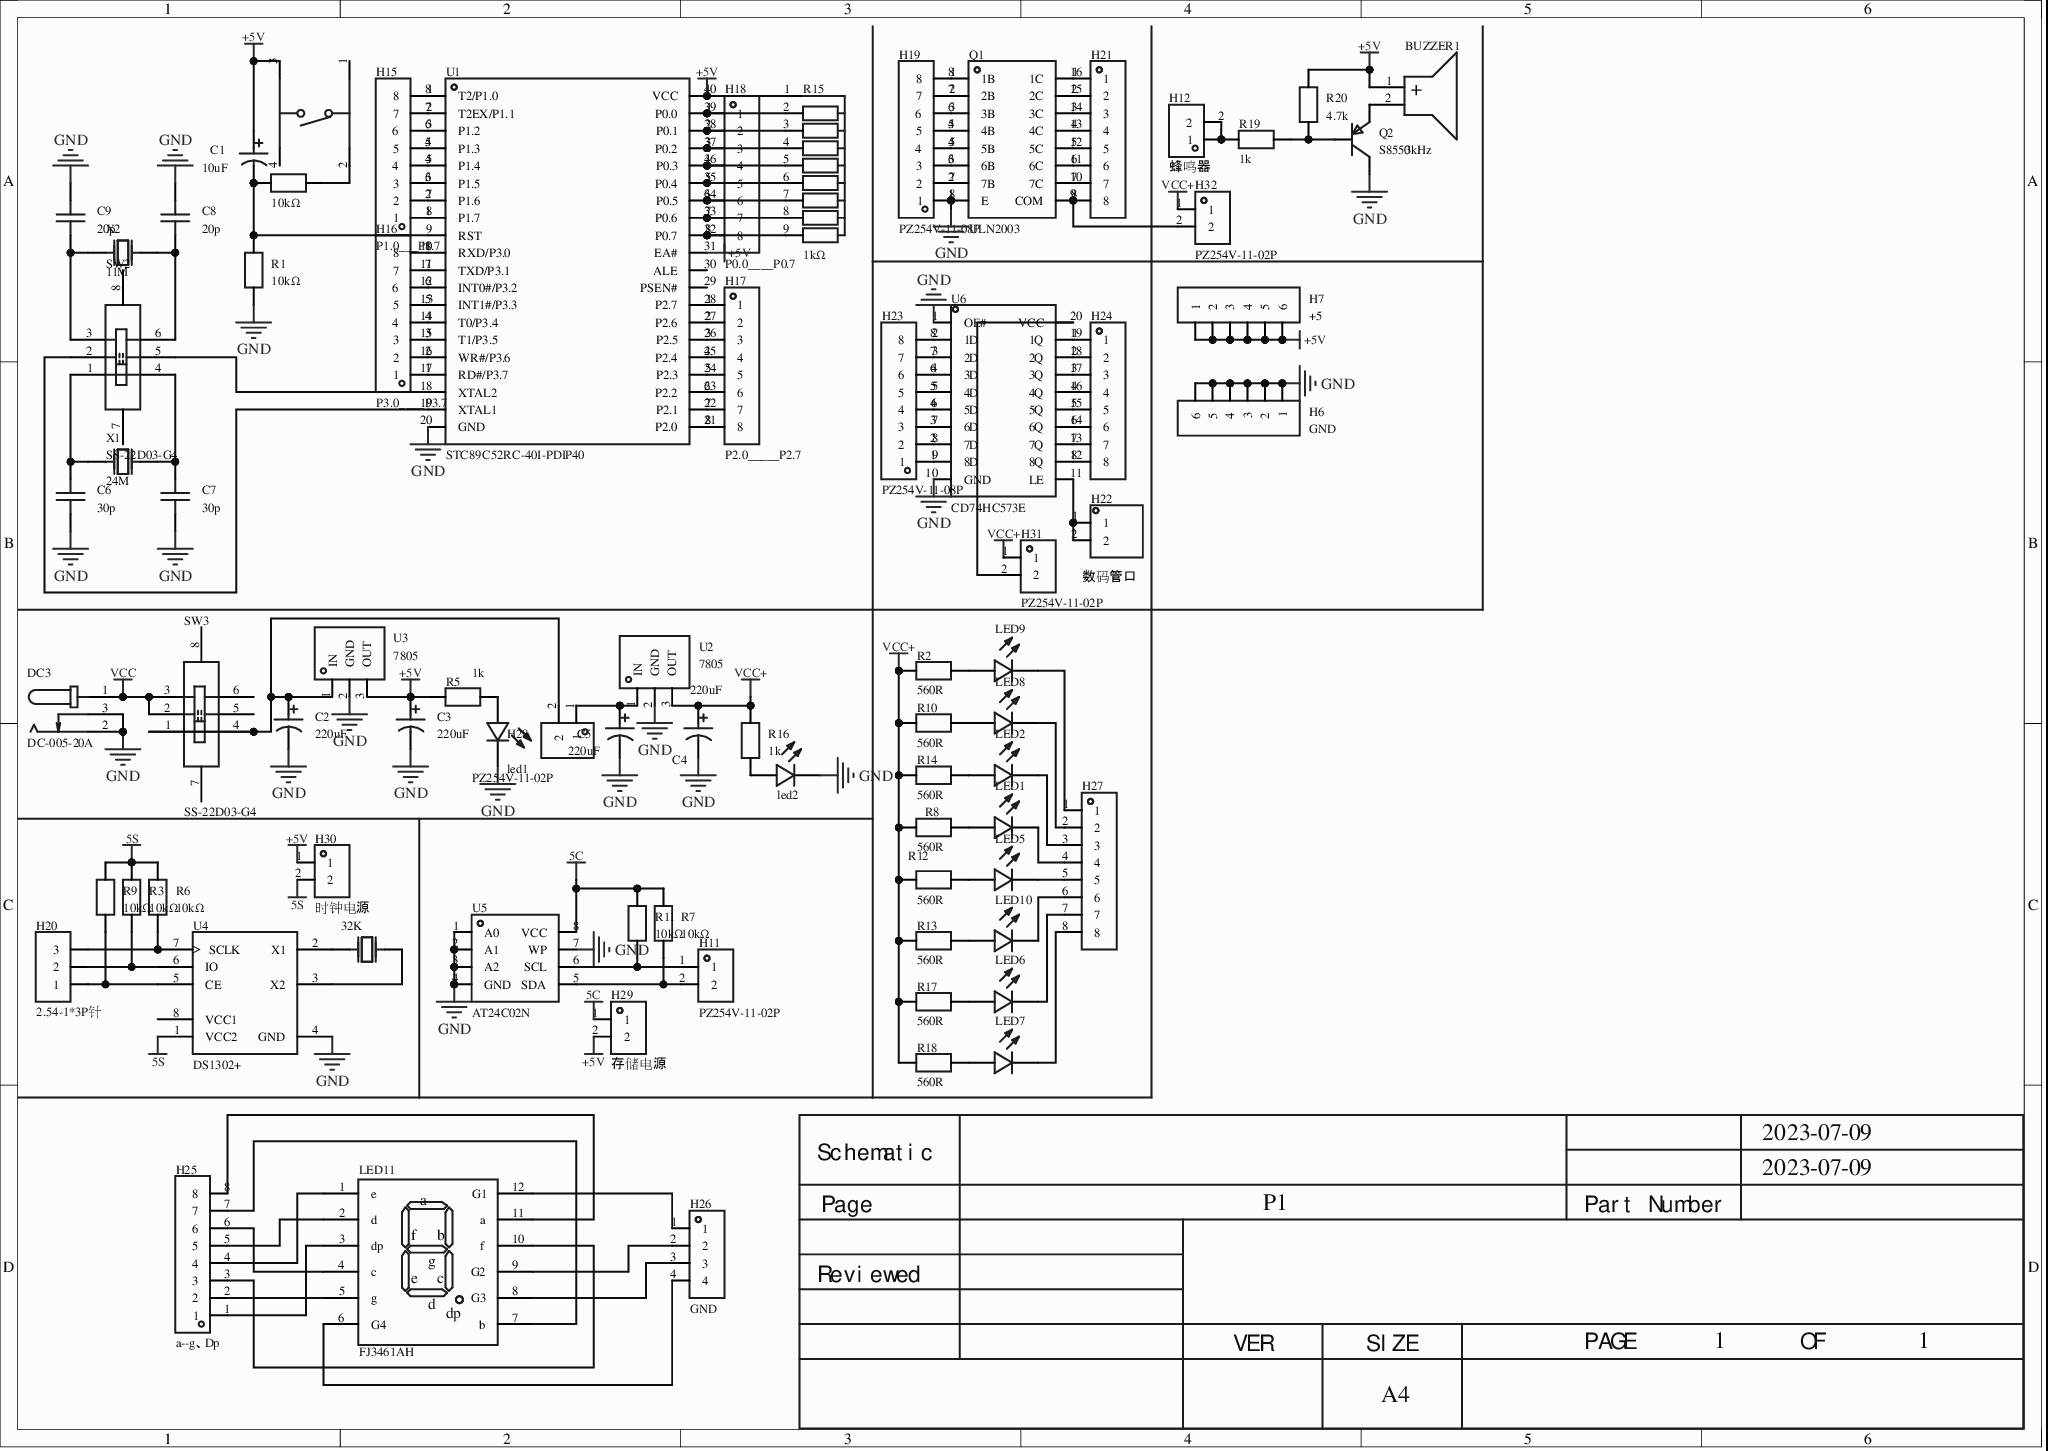
[diagram p0: MISC49922-3.schdoc]
# Altium project MISC49922-2.PrjPcb
1 sheet, 78 parts. Net scope: global (net labels, ports and power ports of the same name join across sheets).
Board file: MISC49922.pcbdoc

## Sheet MISC49922-3.schdoc
size 297 x 210 mm; Version: V1.0; @Project Name: MISC49922; @Page Count: 1; @Update Date: 2023-07-09; @Create Date: 2023-07-09; @Schematic Name: MISC49922; @Page No: 1

### Parts
BUZZER1  3kHz  [BUZ-TH_BD9.0-P5.00-D0.6-FD]
C1  10uF  [CAP-TH_BD5.0-P2.00-D0.8-FD]
C2  220uF  [CAP-TH_BD8.0-P3.50-D0.6-FD]
C3  220uF  [CAP-TH_BD8.0-P3.50-D0.6-FD]
C4  220uF  [CAP-TH_BD8.0-P3.50-D0.6-FD]
C5  220uF  [CAP-TH_BD8.0-P3.50-D0.6-FD]
C6  30p  [CAP-TH_L5.0-W5.0-P2.54-D1.0]
C7  30p  [CAP-TH_L5.0-W5.0-P2.54-D1.0]
C8  20p  [CAP-TH_L5.0-W5.0-P2.54-D1.0]
C9  20p  [CAP-TH_L5.0-W5.0-P2.54-D1.0]
DC3  DC-005-20A  [DC-IN-TH_DC-005-20A]
H6  GND  [HDR-TH_6P-P2.54-V-M-1]
H7  +5  [HDR-TH_6P-P2.54-V-M-1]
H11  PZ254V-11-02P  [HDR-TH_2P-P2.54-V-M]
H12  蜂鸣器  [HDR-TH_2P-P2.54-V-M]
H15  P1.0___P1.7  [HDR-TH_8P-P2.54-V-M]
H16  P3.0____P3.7  [HDR-TH_8P-P2.54-V-M]
H17  P2.0_____P2.7  [HDR-TH_8P-P2.54-V-M]
H18  P0.0____P0.7  [HDR-TH_8P-P2.54-V-M]
H19  PZ254V-11-08P  [HDR-TH_8P-P2.54-V-M]
H20  2.54-1*3P针  [HDR-TH_3P-P2.54-V-M-1]
H21  PZ254V-11-08P  [HDR-TH_8P-P2.54-V-M]  (value not drawn)
H22  数码管口  [HDR-TH_2P-P2.54-V-M-1]
H23  PZ254V-11-08P  [HDR-TH_8P-P2.54-V-M]
H24  PZ254V-11-08P  [HDR-TH_8P-P2.54-V-M]  (value not drawn)
H25  a--g、Dp  [HDR-TH_8P-P2.54-V-M]
H26  GND  [HDR-TH_4P-P2.54-V-M]
H27  PZ254V-11-08P  [HDR-TH_8P-P2.54-V-M]  (value not drawn)
H28  PZ254V-11-02P  [HDR-TH_2P-P2.54-V-M]
H29  存储电源  [HDR-TH_2P-P2.54-V-M]
H30  时钟电源  [HDR-TH_2P-P2.54-V-M]
H31  PZ254V-11-02P  [HDR-TH_2P-P2.54-V-M]
H32  PZ254V-11-02P  [HDR-TH_2P-P2.54-V-M]
LED1  204-10SURD/S530-A3-L  [LED-TH_BD3.0-P2.54-FD]  (value not drawn)
LED2  204-10SURD/S530-A3-L  [LED-TH_BD3.0-P2.54-FD]  (value not drawn)
LED3  led1  [LED-TH_BD3.0-P2.54-FD]
LED4  led2  [LED-TH_BD3.0-P2.54-FD]
LED5  204-10SURD/S530-A3-L  [LED-TH_BD3.0-P2.54-FD]  (value not drawn)
LED6  204-10SURD/S530-A3-L  [LED-TH_BD3.0-P2.54-FD]  (value not drawn)
LED7  204-10SURD/S530-A3-L  [LED-TH_BD3.0-P2.54-FD]  (value not drawn)
LED8  204-10SURD/S530-A3-L  [LED-TH_BD3.0-P2.54-FD]  (value not drawn)
LED9  204-10SURD/S530-A3-L  [LED-TH_BD3.0-P2.54-FD]  (value not drawn)
LED10  204-10SURD/S530-A3-L  [LED-TH_BD3.0-P2.54-FD]  (value not drawn)
LED11  FJ3461AH  [LED-SEG-TH_12P-L30.0-W14.0-P2.54-S10.16-BL]
Q1  ULN2003  [DIP-16_L19.8-W6.5-P2.54-LS7.6-BL]
Q2  S8550  [TO-92-3_L4.9-W3.7-P1.27-L]
R1  10kΩ  [RES-TH_BD2.4-L6.3-P10.30-D0.6]
R2  560R  [RES-TH_BD2.4-L6.3-P10.30-D0.6]
R3  10kΩ  [RES-TH_BD2.4-L6.3-P10.30-D0.6]
R4  10kΩ  [RES-TH_BD2.4-L6.3-P10.30-D0.6]
R5  1k  [RES-TH_BD2.4-L6.3-P10.30-D0.6]
R6  10kΩ  [RES-TH_BD2.4-L6.3-P10.30-D0.6]
R7  10kΩ  [RES-TH_BD2.4-L6.3-P10.30-D0.6]
R8  560R  [RES-TH_BD2.4-L6.3-P10.30-D0.6]
R9  10kΩ  [RES-TH_BD2.4-L6.3-P10.30-D0.6]
R10  560R  [RES-TH_BD2.4-L6.3-P10.30-D0.6]
R11  10kΩ  [RES-TH_BD2.4-L6.3-P10.30-D0.6]
R12  560R  [RES-TH_BD2.4-L6.3-P10.30-D0.6]
R13  560R  [RES-TH_BD2.4-L6.3-P10.30-D0.6]
R14  560R  [RES-TH_BD2.4-L6.3-P10.30-D0.6]
R15  1kΩ  [RES-ARRAY-TH_9P-L22.8-W3.00-P2.54]
R16  1k  [RES-TH_BD2.4-L6.3-P10.30-D0.6]
R17  560R  [RES-TH_BD2.4-L6.3-P10.30-D0.6]
R18  560R  [RES-TH_BD2.4-L6.3-P10.30-D0.6]
R19  1k  [RES-TH_BD2.4-L6.3-P10.30-D0.6]
R20  4.7k  [RES-TH_BD2.4-L6.3-P10.30-D0.6]
SW1  TS-1095-A7B2-D1  [SW-TH_4P-L6.0-W6.0-P4.50-LS6.5]  (value not drawn)
SW2  SS-22D03-G4  [SW-TH_SS-22D03-G4]
SW3  SS-22D03-G4  [SW-TH_SS-22D03-G4]
U1  STC89C52RC-40I-PDIP40  [DIP-40_L52.0-W13.7-P2.54-LS15.2-BL]
U2  7805  [TO-220-3_L10.0-W4.5-P2.54-L]
U3  7805  [TO-220-3_L10.0-W4.5-P2.54-L]
U4  DS1302+  [DIP-8_L9.8-W6.6-P2.54-LS7.6-BL]
U5  AT24C02N  [DIP-8_L9.2-W6.3-P2.54-LS7.62-BL]
U6  CD74HC573E  [DIP-20_L26.8-W6.4-P2.54-LS7.6-BL]
X1  24M  [HC-49US_L11.5-W4.5-P4.88]
X2  11M  [HC-49US_L11.5-W4.5-P4.88]
X3  32K  [HC-49US_L11.5-W4.5-P4.88]

### Nets
5C: H29.1 R7.2 R11.2 U5.8(VCC)
5S: H30.2 R3.2 R6.2 R9.2 U4.1(VCC2)
+5V: BUZZER1.1(+) C1.1 C3.1 H7.1 H7.2 H7.3 H7.4 H7.5 H7.6 H29.2 H30.1 R5.1 R15.1 R20.2 SW1.3 U1.31(EA#) U1.40(VCC) U3.3(OUT)
GND: C2.2 C3.2 C4.2 C5.2 C6.1 C7.1 C8.2 C9.1 DC3.2 DC3.3 H6.1 H6.2 H6.3 H6.4 H6.5 H6.6 H19.1 LED3.2(K) LED4.2(K) Q1.8(E) Q2.3(C) R1.1 U1.20(GND) U2.2(GND) U3.2(GND) U4.4(GND) U5.1(A0) U5.2(A1) U5.3(A2) U5.4(GND) U5.7(WP) U6.1(OE#) U6.10(GND)
VCC: DC3.1 SW3.2 SW3.3
VCC+: C4.1 H31.1 H32.1 R2.1 R8.1 R10.1 R12.1 R13.1 R14.1 R16.2 R17.1 R18.1 U2.3(OUT)
NetBUZZER1_2: BUZZER1.2(-) Q2.1(E)
NetC1_2: C1.2 R1.2 R4.1 U1.9(RST)
NetC2_1: C2.1 H28.2 SW3.1 SW3.4 U3.1(IN)
NetC5_1: C5.1 H28.1 U2.1(IN)
NetC6_2: C6.2 SW2.1 X1.2(OSC2)
NetC7_2: C7.2 SW2.4 X1.1(OSC1)
NetC8_1: C8.1 SW2.6 X2.2(OSC2)
NetC9_2: C9.2 SW2.3 X2.1(OSC1)
NetH11_1: H11.1 R11.1 U5.6(SCL)
NetH11_2: H11.2 R7.1 U5.5(SDA)
NetH12_1: H12.1 H12.2 R19.1
NetH15_1: H15.1 U1.8(P1.7)
NetH15_2: H15.2 U1.7(P1.6)
NetH15_3: H15.3 U1.6(P1.5)
NetH15_4: H15.4 U1.5(P1.4)
NetH15_5: H15.5 U1.4(P1.3)
NetH15_6: H15.6 U1.3(P1.2)
NetH15_7: H15.7 U1.2(T2EX/P1.1)
NetH15_8: H15.8 U1.1(T2/P1.0)
NetH16_1: H16.1 U1.17(RD#/P3.7)
NetH16_2: H16.2 U1.16(WR#/P3.6)
NetH16_3: H16.3 U1.15(T1/P3.5)
NetH16_4: H16.4 U1.14(T0/P3.4)
NetH16_5: H16.5 U1.13(INT1#/P3.3)
NetH16_6: H16.6 U1.12(INT0#/P3.2)
NetH16_7: H16.7 U1.11(TXD/P3.1)
NetH16_8: H16.8 U1.10(RXD/P3.0)
NetH17_1: H17.1 U1.28(P2.7)
NetH17_2: H17.2 U1.27(P2.6)
NetH17_3: H17.3 U1.26(P2.5)
NetH17_4: H17.4 U1.25(P2.4)
NetH17_5: H17.5 U1.24(P2.3)
NetH17_6: H17.6 U1.23(P2.2)
NetH17_7: H17.7 U1.22(P2.1)
NetH17_8: H17.8 U1.21(P2.0)
NetH18_1: H18.1 R15.2 U1.39(P0.0)
NetH18_2: H18.2 R15.3 U1.38(P0.1)
NetH18_3: H18.3 R15.4 U1.37(P0.2)
NetH18_4: H18.4 R15.5 U1.36(P0.3)
NetH18_5: H18.5 R15.6 U1.35(P0.4)
NetH18_6: H18.6 R15.7 U1.34(P0.5)
NetH18_7: H18.7 R15.8 U1.33(P0.6)
NetH18_8: H18.8 R15.9 U1.32(P0.7)
NetH19_2: H19.2 Q1.7(7B)
NetH19_3: H19.3 Q1.6(6B)
NetH19_4: H19.4 Q1.5(5B)
NetH19_5: H19.5 Q1.4(4B)
NetH19_6: H19.6 Q1.3(3B)
NetH19_7: H19.7 Q1.2(2B)
NetH19_8: H19.8 Q1.1(1B)
NetH20_1: H20.1 R9.1 U4.5(CE)
NetH20_2: H20.2 R3.1 U4.6(IO)
NetH20_3: H20.3 R6.1 U4.7(SCLK)
NetH21_1: H21.1 Q1.16(1C)
NetH21_2: H21.2 Q1.15(2C)
NetH21_3: H21.3 Q1.14(3C)
NetH21_4: H21.4 Q1.13(4C)
NetH21_5: H21.5 Q1.12(5C)
NetH21_6: H21.6 Q1.11(6C)
NetH21_7: H21.7 Q1.10(7C)
NetH21_8: H21.8 H32.2 Q1.9(COM)
NetH22_1: H22.1 H22.2 U6.11(LE)
NetH23_1: H23.1 U6.9(8D)
NetH23_2: H23.2 U6.8(7D)
NetH23_3: H23.3 U6.7(6D)
NetH23_4: H23.4 U6.6(5D)
NetH23_5: H23.5 U6.5(4D)
NetH23_6: H23.6 U6.4(3D)
NetH23_7: H23.7 U6.3(2D)
NetH23_8: H23.8 U6.2(1D)
NetH24_1: H24.1 U6.19(1Q)
NetH24_2: H24.2 U6.18(2Q)
NetH24_3: H24.3 U6.17(3Q)
NetH24_4: H24.4 U6.16(4Q)
NetH24_5: H24.5 U6.15(5Q)
NetH24_6: H24.6 U6.14(6Q)
NetH24_7: H24.7 U6.13(7Q)
NetH24_8: H24.8 U6.12(8Q)
NetH25_1: H25.1 LED11.3(dp)
NetH25_2: H25.2 LED11.5(g)
NetH25_3: H25.3 LED11.10(f)
NetH25_4: H25.4 LED11.1(e)
NetH25_5: H25.5 LED11.2(d)
NetH25_6: H25.6 LED11.4(c)
NetH25_7: H25.7 LED11.7(b)
NetH25_8: H25.8 LED11.11(a)
NetH26_1: H26.1 LED11.12(G1)
NetH26_2: H26.2 LED11.9(G2)
NetH26_3: H26.3 LED11.8(G3)
NetH26_4: H26.4 LED11.6(G4)
NetH27_1: H27.1 LED9.2(K)
NetH27_2: H27.2 LED8.2(K)
NetH27_3: H27.3 LED2.2(K)
NetH27_4: H27.4 LED1.2(K)
NetH27_5: H27.5 LED5.2(K)
NetH27_6: H27.6 LED10.2(K)
NetH27_7: H27.7 LED6.2(K)
NetH27_8: H27.8 LED7.2(K)
NetH31_2: H31.2 U6.20(VCC)
NetLED1_1: LED1.1(A) R8.2
NetLED2_1: LED2.1(A) R14.2
NetLED3_1: LED3.1(A) R5.2
NetLED4_1: LED4.1(A) R16.1
NetLED5_1: LED5.1(A) R12.2
NetLED6_1: LED6.1(A) R17.2
NetLED7_1: LED7.1(A) R18.2
NetLED8_1: LED8.1(A) R10.2
NetLED9_1: LED9.1(A) R2.2
NetLED10_1: LED10.1(A) R13.2
NetQ2_2: Q2.2(B) R19.2 R20.1
NetR4_2: R4.2 SW1.2
NetSW2_2: SW2.2 U1.19(XTAL1)
NetSW2_5: SW2.5 U1.18(XTAL2)
NetU4_2: U4.2(X1) X3.2(OSC2)
NetU4_3: U4.3(X2) X3.1(OSC1)

Not connected (* = marked no-connect by the designer): SW1 1* 4*; SW2 7* 8*; SW3 5* 6* 7* 8*; U1 29(PSEN#) 30(ALE); U4 8(VCC1)*

### Notes on the sheet
- 2023-07-09
- Schematic
- Page
- P1
- Part Number
- Reviewed
- VER
- SIZE
- A4
- PAGE
- 1
- OF

### Library data of the parts
BUZZER1 = HNB09A03: 驱动方式:有源(内含驱动线路);构造类型:电磁式;额定电压:3V;工作电压:1.5V~4.5V;消耗电流:30mA;频率:3kHz;声压(SPL):85dB@10cm;直径(φD):9mm;长度:-;宽度:-;高度:5.5mm;工作温度:-20℃~+70℃;; Manufacturer: 华能; AddInBom: yes; ModelId: 13273335caac486e928bafb4d9fdf12d; ModelName: BUZ-TH_D9.0-H5.5-P5.0; ModelTransform: 354.33,354.33,0,90,0,0,-0.005,0,-177.165; Technology Type: 电磁式; Rated Voltage: 3V; Current Consumption: 30mA; Device: HNB09A03; Symbol: HNB09A03; LCSC Part Name: 电磁式有源一体蜂鸣器HNB09A03; SupplierPart: C96102; ManufacturerPart: HNB09A03; Supplier Footprint: 插件,D=9mm; JLCPCB Part Class: Extended Part; Datasheet: https://atta.szlcsc.com/upload/public/pdf/source/20170522/1495448326172.pdf; Supplier: LCSC; ConvertToPcb: yes; FootprintName: BUZ-TH_BD9.0-P5.00-D0.6-FD; Oscillator Circuit: 有源(内含驱动线路); Operating Voltage: 1.5V~4.5V; Value: 3kHz; Sound Pressure Level (SPL): 85dB@10cm; Diameter (φD): 9mm; Length: -; Width: -; Height: 5.5mm; Operating Temperature: -20℃~+70℃
C1 = ERS1HM100D11OT: 容值:10uF;精度:±20%;额定电压:50V;; Manufacturer: AISHI(艾华集团); AddInBom: yes; ModelId: edeeed87cbc746108d01291548c38636; ModelName: CAP-TH_D5.0×H7.0×P2.0; ModelTransform: 197.091,196.7911,0,0,0,0,0,0,-137.795; Tolerance: ±20%; Rated Voltage: 50V; φD: 5mm; L: 11mm; Lifetime @ Temp: 5000hrs@105℃; Device: ERS1HM100D11OT; Symbol: ERS1HM100D11OT; LCSC Part Name: 10uF ±20% 50V; SupplierPart: C106654; ManufacturerPart: ERS1HM100D11OT; Supplier Footprint: 插件,D5xL11mm; JLCPCB Part Class: Extended Part; Datasheet: https://atta.szlcsc.com/upload/public/pdf/source/20170415/1492238168696.pdf; Supplier: LCSC; ConvertToPcb: yes; FootprintName: CAP-TH_BD5.0-P2.00-D0.8-FD; Value: 10uF; Lead Spacing: 2mm
C2-C5 = KM227M035F12RR0VH2FP0: 容值:220uF;精度:±20%;额定电压:35V;纹波电流:-;等效串联电阻:-;; Manufacturer: CX(承兴); Symbol: 220uf/35V; AddInBom: yes; ModelId: a2c936ec27754f809f3966430e36f767; ModelName: CAP-TH_D8.0-H8.0-P3.50; ModelTransform: 314.96,314.862,0,180,0,0,0,0,-137.795; Tolerance: ±20%; Rated Voltage: 35V; φD: 8mm; L: 12mm; Lifetime @ Temp: 2000hrs@105℃; Device: KM227M035F12RR0VH2FP0; LCSC Part Name: 220uF ±20% 35V; SupplierPart: C2063; ManufacturerPart: KM227M035F12RR0VH2FP0; Supplier Footprint: 插件,D8xL12mm; JLCPCB Part Class: Extended Part; Datasheet: https://atta.szlcsc.com/upload/public/pdf/source/20211027/06D6BA3719C264B639DC286D935D03EA.pdf; Supplier: LCSC; ConvertToPcb: yes; FootprintName: CAP-TH_BD8.0-P3.50-D0.6-FD; Value: 220uF; Lead Spacing: 3.5mm; Ripple Current: -; Equivalent Series Resistance(ESR): -
C6-C9 = CC1H150KA1FDCH4B1000: 容值:15pF;精度:±10%;额定电压:50V;温度系数:NP0;; Manufacturer: Dersonic(德尔创); AddInBom: yes; ModelId: 270ac4fb99bb44cf92c070987eedbe36; ModelName: CAP-TH_BD5.0-W5.0-P2.54; ModelTransform: 196.785,98.425,0,0,0,0,0,0,-137.795; Value: 15pF; Tolerance: ±10%; Voltage Rated: 50V; Temperature Coefficient: NP0; φD: 4.7mm; Body Thickness: 2.2mm; Device: CC1H150KA1FDCH4B1000; Symbol: CC1H150KA1FDCH4B1000; LCSC Part Name: 15pF ±10% 50V; SupplierPart: C377839; ManufacturerPart: CC1H150KA1FDCH4B1000; Supplier Footprint: 插件,P=2.54mm; JLCPCB Part Class: Extended Part; Datasheet: https://atta.szlcsc.com/upload/public/pdf/source/20200826/C377839_F813476F254DE34AC2BD26147C8A608E.pdf; Supplier: LCSC; ConvertToPcb: yes; FootprintName: CAP-TH_L5.0-W5.0-P2.54-D1.0; Lead Spacing: 2.54mm
DC3 = DC-005-20A_C136744: 触点内径:2mm;触点外径:6.4mm;额定电流:500mA;额定电压:30V;; Manufacturer: 韩国韩荣; AddInBom: yes; ModelId: a72b9ca70a994526b1ddd7443b6051df; ModelTransform: 366.141,555.117,0,270,0,0,-135.827,83.661,-161.417; Inside Contact Diameter: 2mm; Outside Contact Diameter: 6.4mm; Current Rating (Max): 500mA; Voltage Rating (Max): 30V; Device: DC-005-20A_C136744; Symbol: DC-005-20A_C136744; LCSC Part Name: DC-005-20A  内芯2.0mm 全铜; SupplierPart: C136744; ManufacturerPart: DC-005-20A; Supplier Footprint: 插件; JLCPCB Part Class: Extended Part; Datasheet: https://atta.szlcsc.com/upload/public/pdf/source/20210810/D1FE451D887B1804F0660F580C4AD849.pdf; Supplier: LCSC; ConvertToPcb: yes; FootprintName: DC-IN-TH_DC-005-20A; ModelName: DC-IN-TH_DC-005-20A
H6 H7 = 2.54-1x6P直针: 排数:单排;总PIN位数:6;间距:2.54mm;插针结构:1x6P;行距:-;安装类型:直插;圆针/方针:方针;额定电流:3A;额定电压:-;配合针长度:-;塑高:-;触头材质:黄铜;触头镀层:-;工作温度范围:-40℃~+105℃;颜色:黑色;; Manufacturer: BOOMELE(博穆精密); Symbol: Header-Male-2.54_1x6; AddInBom: yes; ModelId: 60739dffc9b04830a286435b0fefbd4a; ModelName: HDR2.54-M-LI-1X6P; ModelTransform: 599.999,100,0,0,0,0,0,0,-118.11; Pitch: 2.54mm; Pin Structure: 1x6P; Circluar Pins/Square Pins: 方针; Current Rating (Max): 3A; Device: 2.54-1x6P直针; LCSC Part Name: 2.54mm 1x6P 直插 方针; SupplierPart: C37208; ManufacturerPart: 2.54-1x6P直针; Supplier Footprint: 直插,P=2.54mm; JLCPCB Part Class: Extended Part; Datasheet: https://atta.szlcsc.com/upload/public/pdf/source/20151109/1457707558014.pdf; Supplier: LCSC; ConvertToPcb: yes; FootprintName: HDR-TH_6P-P2.54-V-M-1; Number of Rows: 单排; Number of Pins: 6; Row Spacing: -; Mounting Type: 直插; Voltage Rating (Max): -; Length of Mating Pin: -; Insulation Height: -; Contact Material: 黄铜; Contact Plating: -; Operating Temperature Range: -40℃~+105℃; Color: 黑色
H11 H12 H28-H32 = PZ254V-11-02P: 排数:单排;总PIN位数:2;间距:2.54mm;插针结构:1x2P;行距:-;安装类型:直插;圆针/方针:方针;额定电流:-;额定电压:-;配合针长度:6mm;塑高:2.5mm;端接针长度:3mm;触头材质:黄铜;触头镀层:-;工作温度范围:-40℃~+105℃;颜色:黑色;; Manufacturer: XFCN(兴飞); AddInBom: yes; ModelId: e35305ec3aa84b66b849f914b715e73f; ModelName: HDR2.54-M-LI-1X2P; ModelTransform: 200,100,0,0,0,0,0,0,-118.11; Pitch: 2.54mm; Pin Structure: 1x2P; Circluar Pins/Square Pins: 方针; Device: PZ254V-11-02P; Symbol: PZ254V-11-02P; LCSC Part Name: 2.54mm 1x2P 直插 方针; SupplierPart: C492401; ManufacturerPart: PZ254V-11-02P; Supplier Footprint: 直插,P=2.54mm; JLCPCB Part Class: Extended Part; Datasheet: https://atta.szlcsc.com/upload/public/pdf/source/20200309/C492401_A812433581A9B211A7FFA413ADDFF0E5.pdf; Supplier: LCSC; ConvertToPcb: yes; FootprintName: HDR-TH_2P-P2.54-V-M; Number of Rows: 单排; Number of Pins: 2; Row Spacing: -; Mounting Type: 直插; Current Rating (Max): -; Voltage Rating (Max): -; Length of Mating Pin: 6mm; Insulation Height: 2.5mm; Length of End Connection Pin: 3mm; Contact Material: 黄铜; Contact Plating: -; Operating Temperature Range: -40℃~+105℃; Color: 黑色
H15-H19 H21 H23-H25 H27 = PZ254V-11-08P: 排数:单排;总PIN位数:8;间距:2.54mm;插针结构:1x8P;行距:-;安装类型:直插;圆针/方针:方针;额定电流:-;额定电压:-;配合针长度:6mm;塑高:2.5mm;端接针长度:3mm;触头材质:黄铜;触头镀层:-;工作温度范围:-40℃~+105℃;颜色:黑色;; Manufacturer: XFCN(兴飞); AddInBom: yes; ModelId: f5b96e27511e49e38545e53df2320202; ModelTransform: 807.87244,98.425,0,0,0,0,0,0,-118.11; Pitch: 2.54mm; Pin Structure: 1x8P; Circluar Pins/Square Pins: 方针; Device: PZ254V-11-08P; Symbol: PZ254V-11-08P; LCSC Part Name: 2.54mm 1x8P 直插 方针; SupplierPart: C492407; ManufacturerPart: PZ254V-11-08P; Supplier Footprint: 直插,P=2.54mm; JLCPCB Part Class: Extended Part; Datasheet: https://atta.szlcsc.com/upload/public/pdf/source/20200309/C492407_83A6FB26A2233368EDB9516968EC6149.pdf; Supplier: LCSC; ConvertToPcb: yes; FootprintName: HDR-TH_8P-P2.54-V-M; ModelName: HDR-TH_8P-P2.54-V-M; Number of Rows: 单排; Number of Pins: 8; Row Spacing: -; Mounting Type: 直插; Current Rating (Max): -; Voltage Rating (Max): -; Length of Mating Pin: 6mm; Insulation Height: 2.5mm; Length of End Connection Pin: 3mm; Contact Material: 黄铜; Contact Plating: -; Operating Temperature Range: -40℃~+105℃; Color: 黑色
H20 = 2.54-1*3P针: 排数:单排;总PIN位数:3;间距:2.54mm;插针结构:1x3P;行距:-;安装类型:直插;圆针/方针:方针;额定电流:3A;额定电压:-;配合针长度:-;塑高:-;端接针长度:-;触头材质:-;触头镀层:-;工作温度范围:-40℃~+105℃;颜色:黑色;; Manufacturer: BOOMELE(博穆精密); Symbol: Header-Male-2.54_1x3; AddInBom: yes; ModelId: 94a8ffe137b6410295cb18cd3ffd99db; ModelName: HDR-M-2.54_1x3; ModelTransform: 299.9994,100,0,0,0,0,0,0,-118.11; Pitch: 2.54mm; Pin Structure: 1x3P; Circluar Pins/Square Pins: 方针; Current Rating (Max): 3A; Device: 2.54-1*3P针; LCSC Part Name: 2.54mm 1x3P 直插 方针; SupplierPart: C49257; ManufacturerPart: 2.54-1*3P针; Supplier Footprint: 插件,P=2.54mm; JLCPCB Part Class: Extended Part; Datasheet: https://atta.szlcsc.com/upload/public/pdf/source/20221018/3E9408392E35E6F57A28985E5F7BF5C9.pdf; Supplier: LCSC; ConvertToPcb: yes; FootprintName: HDR-TH_3P-P2.54-V-M-1; Number of Rows: 单排; Number of Pins: 3; Row Spacing: -; Mounting Type: 直插; Voltage Rating (Max): -; Length of Mating Pin: -; Insulation Height: -; Length of End Connection Pin: -; Contact Material: -; Contact Plating: -; Operating Temperature Range: -40℃~+105℃; Color: 黑色
H22 = B-2100S02P-A110: 排数:单排;总PIN位数:2;间距:2.54mm;插针结构:1x2P;行距:-;安装类型:直插;圆针/方针:-;额定电流:-;额定电压:-;配合针长度:6mm;塑高:2.54mm;端接针长度:3mm;触头材质:黄铜;触头镀层:-;工作温度范围:-40℃~+105℃;颜色:黑色;; Manufacturer: Ckmtw(灿科盟); Symbol: 210S-1*2P L=11.6MMGold-plated black; AddInBom: yes; ModelId: 79b2e9f2d70a4d68a1b7098f27c6d4c5; ModelName: HDR-M-2.54_1x2; ModelTransform: 200,100,0,0,0,0,0,0,-118.11; Pitch: 2.54mm; Pin Structure: 1x2P; Device: B-2100S02P-A110; LCSC Part Name: 2.54mm 1x2P 直插; SupplierPart: C124375; ManufacturerPart: B-2100S02P-A110; Supplier Footprint: 插件,P=2.54mm; JLCPCB Part Class: Extended Part; Datasheet: https://atta.szlcsc.com/upload/public/pdf/source/20221019/2EE72DAC61CAA62C0A53546E211F9C15.pdf; Supplier: LCSC; ConvertToPcb: yes; FootprintName: HDR-TH_2P-P2.54-V-M-1; Number of Rows: 单排; Number of Pins: 2; Row Spacing: -; Mounting Type: 直插; Circluar Pins/Square Pins: -; Current Rating (Max): -; Voltage Rating (Max): -; Length of Mating Pin: 6mm; Insulation Height: 2.54mm; Length of End Connection Pin: 3mm; Contact Material: 黄铜; Contact Plating: -; Operating Temperature Range: -40℃~+105℃; Color: 黑色
H26 = PZ254V-11-04P: 排数:单排;总PIN位数:4;间距:2.54mm;插针结构:1x4P;行距:-;安装类型:直插;圆针/方针:方针;额定电流:3A;额定电压:250V;配合针长度:6mm;塑高:2.5mm;端接针长度:3mm;触头材质:-;工作温度范围:-40℃~+105℃;颜色:黑色;; Manufacturer: XFCN(兴飞); Symbol: PZ254V-11-04P_C2691448; AddInBom: yes; ModelId: 112f4d05e8d64e99ab9a333894bea4f9; ModelName: HDR-TH_4P-P2.54-M-LI-1X4P; ModelTransform: 399.999,104.7242,0,0,0,0,0,0,-118.11; Pitch: 2.54mm; Pin Structure: 1x4P; Circluar Pins/Square Pins: 方针; Current Rating (Max): 3A; Voltage Rating (Max): 250V; Device: PZ254V-11-04P; LCSC Part Name: 2.54mm 1x4P 直插 方针; SupplierPart: C2691448; ManufacturerPart: PZ254V-11-04P; Supplier Footprint: 直插,P=2.54mm; JLCPCB Part Class: Extended Part; Datasheet: https://atta.szlcsc.com/upload/public/pdf/source/20200309/C492403_F9F19131791D08044AD4F84F8E751A34.pdf; Supplier: LCSC; ConvertToPcb: yes; FootprintName: HDR-TH_4P-P2.54-V-M; Number of Rows: 单排; Number of Pins: 4; Row Spacing: -; Mounting Type: 直插; Length of Mating Pin: 6mm; Insulation Height: 2.5mm; Length of End Connection Pin: 3mm; Contact Material: -; Operating Temperature Range: -40℃~+105℃; Color: 黑色
LED1-LED10 = 204-10SURD/S530-A3-L: 发光颜色:红灯;二极管配置:-;主波长:624nm;色温:-;功率:60mW;安装方式:-;; Manufacturer: EVERLIGHT(亿光); AddInBom: yes; ModelId: a497c992633541038a38947cdc58012f; ModelName: LED-TH-3mm_R; ModelTransform: 141.274,153.327,0,0,0,0,-5.984,0,-137.795; Emitted Color: 红灯; Lens Color: 雾状红; Dominant Wavelength: 624nm; Peak Wavelength: 632nm; Forward Current: 20mA; Power Dissipation: 60mW; Viewing Angle: 40°; Lamp Holder Type: 3mm圆形灯头; Device: 204-10SURD/S530-A3-L; Symbol: 204-10SURD/S530-A3-L; LCSC Part Name: 红灯; SupplierPart: C99771; ManufacturerPart: 204-10SURD/S530-A3-L; Supplier Footprint: 插件,D=3mm; JLCPCB Part Class: Extended Part; Datasheet: https://atta.szlcsc.com/upload/public/pdf/source/20170504/1493866972127.pdf; Supplier: LCSC; ConvertToPcb: yes; FootprintName: LED-TH_BD3.0-P2.54-FD; Diode Configuration: -; Color Temperature: -; Mounting Sytle: -; Operating Temperature: -40℃~+85℃
LED11 = FJ3461AH: 数码管位数:4;数字/字母大小(英寸):0.36;LED极性:共阴;发光颜色:红色;; Manufacturer: 志浩; AddInBom: yes; ModelId: 413f3531b06c40ffa975bee3b430fbb4; ModelName: LED-SEG-TH_0.36-4P; ModelTransform: 1181.1,551.18,0,0,0,0,-0.001,-0.001,-137.795; Number of Characters: 4; Digit/Alpha Size(inch): 0.36; LED Polarity: 共阴; Luminous Color: 红色; Module Size: 30mmx14mmx7.2mm; Device: FJ3461AH; Symbol: FJ3461AH; LCSC Part Name: 4位0.36英寸红色数码管 共阴极; SupplierPart: C10708; ManufacturerPart: FJ3461AH; Supplier Footprint: 插件; JLCPCB Part Class: Extended Part; Datasheet: https://atta.szlcsc.com/upload/public/pdf/source/20121231/1457706574766.pdf; Supplier: LCSC; ConvertToPcb: yes; FootprintName: LED-SEG-TH_12P-L30.0-W14.0-P2.54-S10.16-BL; Display Type: -; Power Dissipation: -
Q1 = ULN2003_C557872: Manufacturer: YW(友旺); AddInBom: yes; ModelId: 1d8537d07c784a01867ee00a159e9dcc; ModelName: DIP-16_L20.0-W6.4-H3.5-LS7.62-P2.54; ModelTransform: 787.4,311.8104,0,0,0,0,-0.003,0.001,-118.11; Device: ULN2003_C557872; Symbol: ULN2003_C557872; LCSC Part Name: 七路达林顿晶体管阵列; SupplierPart: C557872; ManufacturerPart: ULN2003; Supplier Footprint: DIP-16; JLCPCB Part Class: Extended Part; Datasheet: https://atta.szlcsc.com/upload/public/pdf/source/20200527/C557873_2AFF25600AE9CE704FFBA5741FE31C9F.pdf; Supplier: LCSC; ConvertToPcb: yes; FootprintName: DIP-16_L19.8-W6.5-P2.54-LS7.6-BL
Q2 = S8550_C717454: 晶体管类型:PNP;集射极击穿电压(Vceo):25V;集电极电流(Ic):500mA;功率(Pd):625mW;集电极截止电流(Icbo):100nA;集电极-发射极饱和电压(VCE(sat)@Ic,Ib):600mV@500mA,50mA;特征频率(fT):150MHz;工作温度:-55℃~+150℃@(Tj);; Manufacturer: LGE(鲁光); AddInBom: yes; ModelId: aafe8e06f2154e7c93506efd0d6632dd; ModelTransform: 180.7872,141.4455,0,0,0,0,0,22.677,-196.85; Transistor Type: PNP; Collector-Emitter Breakdown Voltage (Vceo): 25V; Collector Current (Ic): 500mA; Power Dissipation (Pd): 625mW; Collector Cut-Off Current (Icbo): 100nA; Transition Frequency (fT): 150MHz; Device: S8550_C717454; Symbol: S8550_C717454; LCSC Part Name: PNP 25V 500mA; SupplierPart: C717454; ManufacturerPart: S8550; Supplier Footprint: TO-92; JLCPCB Part Class: Extended Part; Datasheet: https://atta.szlcsc.com/upload/public/pdf/source/20200803/C717454_33122355B4D3E5923B6EDC09959755A6.pdf; Supplier: LCSC; ConvertToPcb: yes; FootprintName: TO-92-3_L4.9-W3.7-P1.27-L; ModelName: TO-92-3_L4.9-W3.7-P1.27-L; Collector-Emitter Saturation Voltage (VCE(sat)@Ic,Ib): 600mV@500mA,50mA; Operating Temperature: -55℃~+150℃@(Tj)
R1 R3 R4 R6 R7 R9 R11 = RN1/4W10KFT/BA1: 电阻类型:金属膜电阻;阻值:10kΩ;精度:±1%;功率:250mW;温度系数:±50ppm/℃;最大工作电压:250V;工作温度范围:-55℃~+125℃;; Manufacturer: Tyohm(幸亚电阻); AddInBom: yes; ModelId: 463263665006444ab7a47bd11b0cf956; ModelTransform: 427.165,94.32816,0,0,0,0,0,0,-196.85; Tolerance: ±1%; Power(Watts): 250mW; Overload Voltage (Max): 250V; Device: RN1/4W10KFT/BA1; Symbol: RN 1/4W 10K F T/B A1; LCSC Part Name: 金属膜电阻 10kΩ ±1% 250mW; SupplierPart: C410695; ManufacturerPart: RN1/4W10KFT/BA1; Supplier Footprint: 插件; JLCPCB Part Class: Extended Part; Datasheet: https://atta.szlcsc.com/upload/public/pdf/source/20190808/C410695_F4C96186075092C4BC649A77CE7E5B2A.pdf; Supplier: LCSC; ConvertToPcb: yes; FootprintName: RES-TH_BD2.4-L6.3-P10.30-D0.6; ModelName: RES-TH_BD2.4-L6.3-P10.30-D0.6; Type: 金属膜电阻; Value: 10kΩ; Temperature Coefficient: ±50ppm/℃; Operating Temperature Range: -55℃~+125℃
R2 R5 R8 R10 R12-R14 R16-R20 = RN1/4W10KFT/BA1: 电阻类型:金属膜电阻;阻值:10kΩ;精度:±1%;功率:250mW;温度系数:±50ppm/℃;最大工作电压:250V;工作温度范围:-55℃~+125℃;; Manufacturer: Tyohm(幸亚电阻); AddInBom: yes; ModelId: 463263665006444ab7a47bd11b0cf956; ModelTransform: 427.165,94.32816,0,0,0,0,0,0,-196.85; Value: 10kΩ; Tolerance: ±1%; Power(Watts): 250mW; Overload Voltage (Max): 250V; Device: RN1/4W10KFT/BA1; Symbol: RN 1/4W 10K F T/B A1; LCSC Part Name: 金属膜电阻 10kΩ ±1% 250mW; SupplierPart: C410695; ManufacturerPart: RN1/4W10KFT/BA1; Supplier Footprint: 插件; JLCPCB Part Class: Extended Part; Datasheet: https://atta.szlcsc.com/upload/public/pdf/source/20190808/C410695_F4C96186075092C4BC649A77CE7E5B2A.pdf; Supplier: LCSC; ConvertToPcb: yes; FootprintName: RES-TH_BD2.4-L6.3-P10.30-D0.6; ModelName: RES-TH_BD2.4-L6.3-P10.30-D0.6; Type: 金属膜电阻; Temperature Coefficient: ±50ppm/℃; Operating Temperature Range: -55℃~+125℃
R15 = 4609X-101-102LF: 阻值:1kΩ;精度:±2%;单个元件功率:200mW;电阻器数:8;; Manufacturer: BOURNS; AddInBom: yes; ModelId: 3a4ef2fe01494457934b8bd09212e327; ModelName: RES-ARRAY-TH_9P-L22.8-W3.00-H5.08-P2.54; ModelTransform: 914.1714,114.13505,0,0,0,0,0,0,-137.795; Tolerance: ±2%; Power(Watts): 200mW; Number of Resistors: 8; Temperature Coefficient: ±100ppm/℃; Device: 4609X-101-102LF; Symbol: 4609X-101-102LF; LCSC Part Name: 1kΩ ±2%; SupplierPart: C840661; ManufacturerPart: 4609X-101-102LF; Supplier Footprint: SIP-9-2.54mm; JLCPCB Part Class: Extended Part; Datasheet: https://atta.szlcsc.com/upload/public/pdf/source/20210602/12BA461036BFCE8593BA6D5AE69068B1.pdf; Supplier: LCSC; ConvertToPcb: yes; FootprintName: RES-ARRAY-TH_9P-L22.8-W3.00-P2.54; Value: 1kΩ; Number of Pins: 9
SW1 = TS-1095-A7B2-D1: 电路结构:单刀单掷;安装方式:直插;作用力:180gf@±30gf;机械寿命:-;带支架:否;; Manufacturer: Yuandi(元迪); AddInBom: yes; ModelId: 20eee248bc684ccd8cbdbb1d0d91ec6f; ModelName: SW-TH_4P-L6.0-W6.0-H5.0-LS6.5-P4.50; ModelTransform: 236.22,323.03,0,90,0,0,0,0,-137.795; Circuit: 单刀单掷; Actuator Style: 圆形按钮; Actuator/Cap Color: 黑色; Pin Style: PC引脚; Switch Length: 6mm; Switch Height: 7mm; Strike Gundam: 否; Device: TS-1095-A7B2-D1; Symbol: TS-1095-A7B2-D1; LCSC Part Name: 6*6*7mm 直插 轻触开关; SupplierPart: C782810; ManufacturerPart: TS-1095-A7B2-D1; Supplier Footprint: 插件; JLCPCB Part Class: Extended Part; Datasheet: https://atta.szlcsc.com/upload/public/pdf/source/20200908/C782804_D14F61DCCBE05C7EE913124CF28857B3.pdf; Supplier: LCSC; ConvertToPcb: yes; FootprintName: SW-TH_4P-L6.0-W6.0-P4.50-LS6.5; Mounting Style: 直插; Operating Force: 180gf@±30gf; Mechanical Life: -; Switch Width: 6mm
SW2 SW3 = SS-22D03-G4_C136717: 额定电流(DC):-;额定电压(DC):-;额定电流(AC):-;额定电压(AC):-;电路结构:单刀双掷;安装方式:直插;机械寿命:5千次;; Manufacturer: 韩国韩荣; AddInBom: yes; ModelId: d5a131114e044d9aa6e65c020ab08784; ModelTransform: 338.58751,271.653,0,0,0,0,0,0,-110.236; Circuit: 单刀双掷; Mechanical Life: 5千次; Actuator Style: 矩形柱状; Pin Style: PC引脚; Switch Height: 8.7mm; Device: SS-22D03-G4_C136717; Symbol: SS-22D03-G4; LCSC Part Name: 直插双档 滑动开关; SupplierPart: C136717; ManufacturerPart: SS-22D03-G4; Supplier Footprint: 插件; JLCPCB Part Class: Extended Part; Datasheet: https://atta.szlcsc.com/upload/public/pdf/source/20171030/C136717_15093664983011068207.pdf; Supplier: LCSC; ConvertToPcb: yes; FootprintName: SW-TH_SS-22D03-G4; ModelName: SW-TH_SS-22D03-G4; Current Rating (DC): -; Voltage Rating (DC): -; Current Rating (AC): -; Voltage Rating (AC): -; Mounting Style: 直插; Operating Temperature: -25℃~+70℃
U1 = STC89C52RC-40I-PDIP40: CPU内核:51系列;CPU最大主频:-;工作电压范围:3.3V~5.5V;内部振荡器:-;外部时钟频率范围:-;程序 FLASH容量:8KB;RAM总容量:512Byte;EEPROM/数据 FLASH容量:4KB;GPIO端口数量:35;ADC(单元数/通道数/位数):-;DAC(单元数/通道数/位数):-;(E)PWM(单元数/通道数/位数):-;8位Timer数量:-;16位Timer数量:3;32位Timer数量:-;内部比较器数量:-;U(S)ART路数:1;I2C路数:-;I2S路数:-;(; Manufacturer: STC(宏晶); AddInBom: yes; ModelId: 16d4686a009b4ddca948f91eddb57b14; ModelName: DIP-40_L52.3-W13.8-H4.0-LS15.24-P2.54; ModelTransform: 2059.051,615.743,0,0,0,0,0,0,-118.11; CPU Core: 51系列; Program FLASH Size: 8KB; EEPROM/Data FLASH Size: 4KB; GPIO Ports Number: 35; 16Bit Timer Number: 3; U(S)ART Number: 1; Peripherals / Functions / Protocol Stacks: 看门狗; Device: STC89C52RC-40I-PDIP40; Symbol: STC89C52RC-40I; LCSC Part Name: 51系列 闪存：8KB RAM：512Byte; SupplierPart: C14022; ManufacturerPart: STC89C52RC-40I-PDIP40; Supplier Footprint: DIP-40; JLCPCB Part Class: Extended Part; Datasheet: https://atta.szlcsc.com/upload/public/pdf/source/20210104/C14022_3E6032FDBB5DBC6F971AD019A8472F5B.pdf; Supplier: LCSC; ConvertToPcb: yes; FootprintName: DIP-40_L52.0-W13.7-P2.54-LS15.2-BL; Maximum Frequency: -; Supply Voltage Range: 3.3V~5.5V; Internal Oscillator: -; External Clock Frequency Rang: -; RAM Size: 512Byte; ADC (Units/Channels/bits): -; DAC (Units/Channels/bits): -; (E)PWM (Units/Channels/bits): -; 8Bit Timer Number: -; 32Bit Timer Number: -; CMP Number: -; I2C Number: -; I2S Number: -; (Q)SPI Number: -; CAN Number: -; USB (H/D/OTG): -; Operating Temperature Range: -40℃~+85℃
U2 U3 = 7805_C2843718: 输出类型:-;; Manufacturer: PUOLOP(迪浦); AddInBom: yes; ModelId: b3c9e38e4428458f8b925050989b538f; ModelTransform: 397.637,177.165,0,180,0,0,-0.004,19.88,-78.74; Device: 7805_C2843718; Symbol: 7805_C2843718; LCSC Part Name: 7805; SupplierPart: C2843718; ManufacturerPart: 7805; Supplier Footprint: TO-220; JLCPCB Part Class: Extended Part; Datasheet: https://atta.szlcsc.com/upload/public/pdf/source/20210712/C2843718_96B9427BF64C6CE0C1AB214F0C19FF34.pdf; Supplier: LCSC; ConvertToPcb: yes; FootprintName: TO-220-3_L10.0-W4.5-P2.54-L; ModelName: TO-220-3_L10.0-W4.5-P2.54-L; Output Type: -
U4 = DS1302+: 3线串行接口，带31个字节RAM，涓流充电，工作电压：2.0V-5.5V; Manufacturer: MAXIM(美信); AddInBom: yes; ModelId: db2af726fcec488f8bf8e467aca974b3; ModelName: DIP-8_L9.8-W6.6-H3.5-LS7.62-P2.54; ModelTransform: 385.826,311.8104,0,0,0,0,-1.693,0,-137.795; Device: DS1302+; Symbol: DS1302+; LCSC Part Name: DS1302; SupplierPart: C14785; ManufacturerPart: DS1302+; Supplier Footprint: DIP-8; JLCPCB Part Class: Extended Part; Datasheet: https://atta.szlcsc.com/upload/public/pdf/source/20130705/1457706621880.pdf; Supplier: LCSC; ConvertToPcb: yes; FootprintName: DIP-8_L9.8-W6.6-P2.54-LS7.6-BL
U5 = AT24C02N: Manufacturer: HGSEMI(华冠); AddInBom: yes; ModelId: 04144a82bcea4a69a3aadaf7b35f2f8c; ModelTransform: 362.204,299.9994,0,0,0,0,0,0,-118.11; Device: AT24C02N; Symbol: AT24C02N; LCSC Part Name: AT24C02N; SupplierPart: C434606; ManufacturerPart: AT24C02N; Supplier Footprint: DIP-8; JLCPCB Part Class: Extended Part; Datasheet: https://atta.szlcsc.com/upload/public/pdf/source/20210719/C565361_F396BA4F8936B5234E7942D8C3C128A6.pdf; Supplier: LCSC; ConvertToPcb: yes; FootprintName: DIP-8_L9.2-W6.3-P2.54-LS7.62-BL; ModelName: DIP-8_L9.2-W6.3-P2.54-LS7.62-BL
U6 = CD74HC573E: 逻辑类型:D型锁存器;电源电压:2V~6V;传播延迟:30ns;; Manufacturer: TI(德州仪器); AddInBom: yes; ModelId: 1b13b515406c47cd93e914408357c80a; ModelName: DIP-20_L26.2-W6.4-H5.4-LS7.62-P2.54; ModelTransform: 1031.494,315.7474,0,0,0,0,0,0,-118.11; Logic Type: D型锁存器; Output Type: 三态; Supply Voltage: 2V~6V; Propagation Delay: 30ns; Sink Current: 7.8mA; Device: CD74HC573E; Symbol: CD74HC573E; LCSC Part Name: 三态输出D型锁存器; SupplierPart: C354058; ManufacturerPart: CD74HC573E; Supplier Footprint: PDIP-20; JLCPCB Part Class: Extended Part; Datasheet: https://atta.szlcsc.com/upload/public/pdf/source/20190124/C354058_C7DF919278C8C5F91192429BB525E9A9.pdf; Supplier: LCSC; ConvertToPcb: yes; FootprintName: DIP-20_L26.8-W6.4-P2.54-LS7.6-BL; Series: 74HC; Source Current: 7.8mA; OperatingTemperature: -55℃~+125℃
X1-X3 = X49SD12MSD2SC: 频率:12MHz;频率公差:±20ppm;频率稳定度:±30ppm;负载电容:20pF;; Manufacturer: YXC(扬兴晶振); AddInBom: yes; ModelId: a8e34f6c394c4d60ace7720f62d1ccdf; ModelName: HC-49US_L11.0-W4.5-H3.5-P4.88; ModelTransform: 432.46488,177.165,0,0,0,0,0,0,-137.795; Crystal Type: 49S晶振; Value: 12MHz; Frequency Tolerance: ±20ppm; Frequency Stability: ±30ppm; Load Capacitance: 20pF; Device: X49SD12MSD2SC; Symbol: X49SD12MSD2SC; LCSC Part Name: 12MHz ±20ppm 内置负载电容:20pF; SupplierPart: C16369; ManufacturerPart: X49SD12MSD2SC; Supplier Footprint: HC-49S; JLCPCB Part Class: Extended Part; Datasheet: https://atta.szlcsc.com/upload/public/pdf/source/20210903/A997D130AE99CBB55D9024F9BE6DA174.pdf; Supplier: LCSC; ConvertToPcb: yes; FootprintName: HC-49US_L11.5-W4.5-P4.88; Operating Temperature: -20℃~+70℃